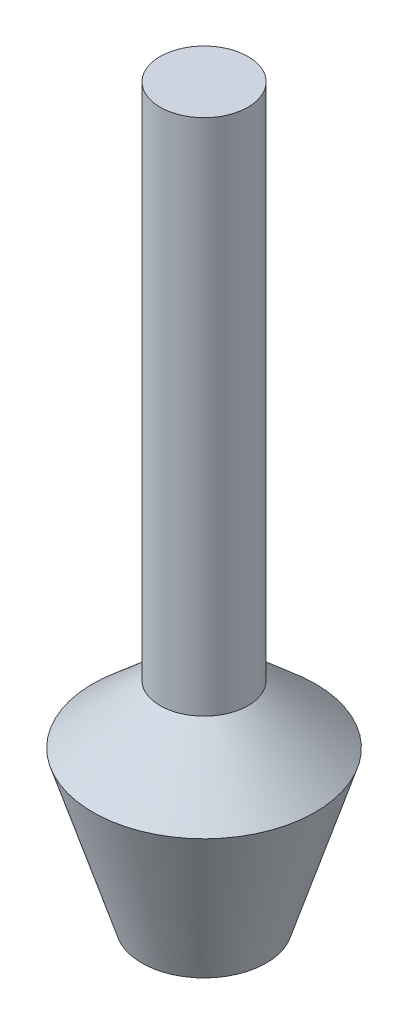
SolidWorks part; units mm, degrees
ref_plane "Plane1" through (0, 0, 0) normal (0, 0, 1) x (1, 0, 0)
ref_plane "Plane2" through (0, 0, 0) normal (0, 1, 0) x (-1, 0, 0)
ref_plane "Plane3" through (0, 0, 0) normal (1, 0, 0) x (0, 0, -1)
sketch "Sketch1" plane through (0, 0, 0) normal (0, 0, 1) x (1, 0, 0)
  line L0 (0, 0) -> (0, 91.3243) construction
  line L1 (3.81, 63.5) -> (3.81, 18.542)
  line L2 (0, 63.5) -> (3.81, 63.5)
  line L3 (0, 0) -> (5.3975, 0)
  line L4 (9.652, 13.462) -> (5.3975, 0)
  line L5 (9.652, 13.462) -> (3.81, 18.542)
  line L6 (0, 63.5) -> (0, 0)
  dimension "D1" = 18.542
  dimension "D2" = 10.795
  dimension "D3" = 19.304
  dimension "D4" = 7.62
  dimension "D5" = 13.462
  dimension "D6" = 63.5
revolve "Base-Revolve" add sketch "Sketch1" angle 360 about L0
